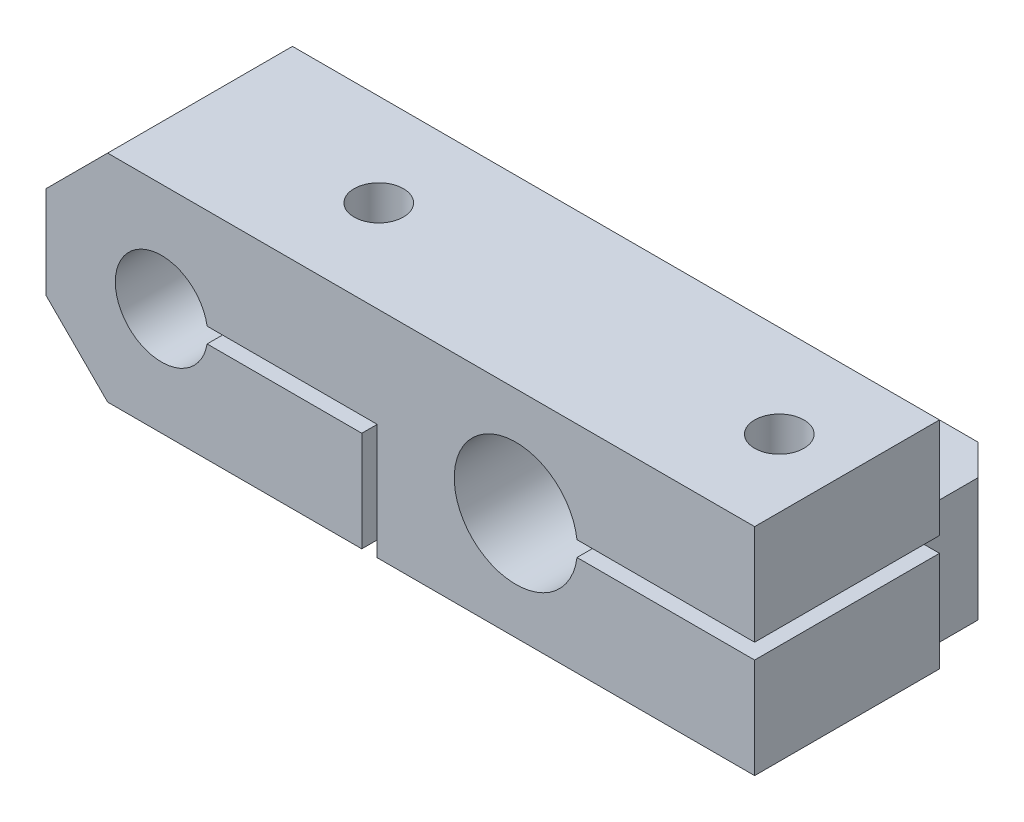
from build123d import *

# Parameters (mm, degrees)
SKETCH1_W           = 29
SKETCH1_H           = 15
SKETCH1_R           = 2
SKETCH1_R_2         = 1.5
BOSS_EXTRUDE1_DEPTH = 13
SKETCH3_W           = 4.75
SKETCH3_H           = 13
SKETCH3_W_2         = 18.25
CUT_EXTRUDE1_DEPTH  = 4
SKETCH5_W           = 29
SKETCH5_H           = 4
CUT_EXTRUDE2_DEPTH  = 27
SKETCH6_W           = 1.5
SKETCH6_H           = 7
CUT_EXTRUDE3_DEPTH  = 27
SKETCH7_W           = 27.5
SKETCH7_H           = 7
CUT_EXTRUDE4_DEPTH  = 7
CHAMFER1_SIZE       = 6
CHAMFER1_SIZE2      = 4
SKETCH8_W           = 6.5
SKETCH8_H           = 0.5
CUT_EXTRUDE5_DEPTH  = 9
SKETCH9_R           = 1.25
CUT_EXTRUDE6_DEPTH  = 3.25
SKETCH12_W          = 3
SKETCH12_H          = 7
CUT_EXTRUDE8_DEPTH  = 8
SKETCH13_R          = 1.5
CUT_EXTRUDE9_DEPTH  = 8
CHAMFER3_SIZE       = 1
SKETCH17_W          = 1.5
SKETCH17_H          = 7
CUT_EXTRUDE11_DEPTH = 9
CHAMFER4_SIZE       = 2
M2_TAPPED_HOLE1_D   = 1.6


with BuildPart() as part:
    # Sketch1 → Boss-Extrude1 (new body)
    with BuildSketch(Plane.XY):
        Rectangle(SKETCH1_W, SKETCH1_H)
        with Locations(Location((6.75, 0, 0), (0, 0, 180))):
            Circle(SKETCH1_R, mode=Mode.SUBTRACT)
        with Locations(Location((-4.75, 0, 0), (0, 0, 180))):
            Circle(SKETCH1_R_2, mode=Mode.SUBTRACT)
    extrude(amount=BOSS_EXTRUDE1_DEPTH)

    # Sketch3 → Cut-Extrude1 (cut)
    with BuildSketch(Plane.XZ.offset(7.5)):
        with Locations((12.125, 6.5)):
            Rectangle(SKETCH3_W, SKETCH3_H)
        with Locations((-5.375, 6.5)):
            Rectangle(SKETCH3_W_2, SKETCH3_H)
    extrude(amount=-CUT_EXTRUDE1_DEPTH, mode=Mode.SUBTRACT)

    # Sketch5 → Cut-Extrude2 (cut)
    with BuildSketch(Plane(origin=(0, 0, 0), x_dir=(-1, 0, 0), z_dir=(0, 0, -1))):
        with Locations((0, 5.5)):
            Rectangle(SKETCH5_W, SKETCH5_H)
    extrude(amount=-CUT_EXTRUDE2_DEPTH, mode=Mode.SUBTRACT)

    # Sketch6 → Cut-Extrude3 (cut)
    with BuildSketch(Plane(origin=(0, 0, 0), x_dir=(-1, 0, 0), z_dir=(0, 0, -1))):
        with Locations((13.75, 0)):
            Rectangle(SKETCH6_W, SKETCH6_H)
    extrude(amount=-CUT_EXTRUDE3_DEPTH, mode=Mode.SUBTRACT)

    # Sketch7 → Cut-Extrude4 (cut)
    with BuildSketch(Plane(origin=(0, 0, 0), x_dir=(-1, 0, 0), z_dir=(0, 0, -1))):
        with Locations((-0.75, 0)):
            Rectangle(SKETCH7_W, SKETCH7_H)
    extrude(amount=-CUT_EXTRUDE4_DEPTH, mode=Mode.SUBTRACT)

    # Chamfer1
    chamfer1_edges = [part.edges().sort_by_distance(p)[0] for p in [
        (6.75, -7.5, 13),
    ]]
    chamfer1_side = [part.faces().sort_by_distance(p)[0] for p in [
        (6.75, -7.5, 6.5),
    ]]
    chamfer(chamfer1_edges, length=CHAMFER1_SIZE, length2=CHAMFER1_SIZE2, reference=chamfer1_side[0])

    # Sketch8 → Cut-Extrude5 (cut)
    with BuildSketch(Plane(origin=(0, 0, 7), x_dir=(-1, 0, 0), z_dir=(0, 0, -1))):
        Polygon((-1.75, -3.5), (-1.75, -0.25), (3.75, -0.25), (3.75, 0.25), (-2.25, 0.25), (-2.25, -3.5), align=None)
        with Locations((-11.25, 0)):
            Rectangle(SKETCH8_W, SKETCH8_H)
    extrude(amount=-CUT_EXTRUDE5_DEPTH, mode=Mode.SUBTRACT)

    # Sketch9 → Cut-Extrude6 (cut)
    with BuildSketch(Plane.XZ.offset(3.5)):
        with Locations((12.3, 10)):
            Circle(SKETCH9_R)
        with Locations((-0.7, 10)):
            Circle(SKETCH9_R)
    extrude(amount=-CUT_EXTRUDE6_DEPTH, mode=Mode.SUBTRACT)

    # Sketch12 → Cut-Extrude8 (cut)
    with BuildSketch(Plane.XY.offset(13)):
        with Locations((-11.5, 0)):
            Rectangle(SKETCH12_W, SKETCH12_H)
    extrude(amount=-CUT_EXTRUDE8_DEPTH, mode=Mode.SUBTRACT)

    # Sketch13 → Cut-Extrude9 (cut)
    with BuildSketch(Plane.XZ.offset(7.5)):
        with Locations((6.75, 3)):
            Circle(SKETCH13_R)
    extrude(amount=-CUT_EXTRUDE9_DEPTH, mode=Mode.SUBTRACT)

    # Chamfer3
    chamfer3_edges = [part.edges().sort_by_distance(p)[0] for p in [
        (9.75, -5.5, 0),
        (3.75, -5.5, 0),
    ]]
    chamfer(chamfer3_edges, length=CHAMFER3_SIZE)

    # Sketch17 → Cut-Extrude11 (cut)
    with BuildSketch(Plane(origin=(0, 0, 7), x_dir=(-1, 0, 0), z_dir=(0, 0, -1))):
        with Locations((9.25, 0)):
            Rectangle(SKETCH17_W, SKETCH17_H)
    extrude(amount=-CUT_EXTRUDE11_DEPTH, mode=Mode.SUBTRACT)

    # Chamfer4
    chamfer4_edges = [part.edges().sort_by_distance(p)[0] for p in [
        (-8.5, -3.5, 10),
        (-8.5, 3.5, 10),
    ]]
    chamfer(chamfer4_edges, length=CHAMFER4_SIZE)

    # M2 Tapped Hole1 (through all)
    with Locations(Plane(origin=(0, 3.5, 0), x_dir=(1, 0, 0), z_dir=(0, 1, 0))):
        with Locations((-0.7, -10), (12.3, -10)):
            Hole(M2_TAPPED_HOLE1_D / 2)


solid = part.part
